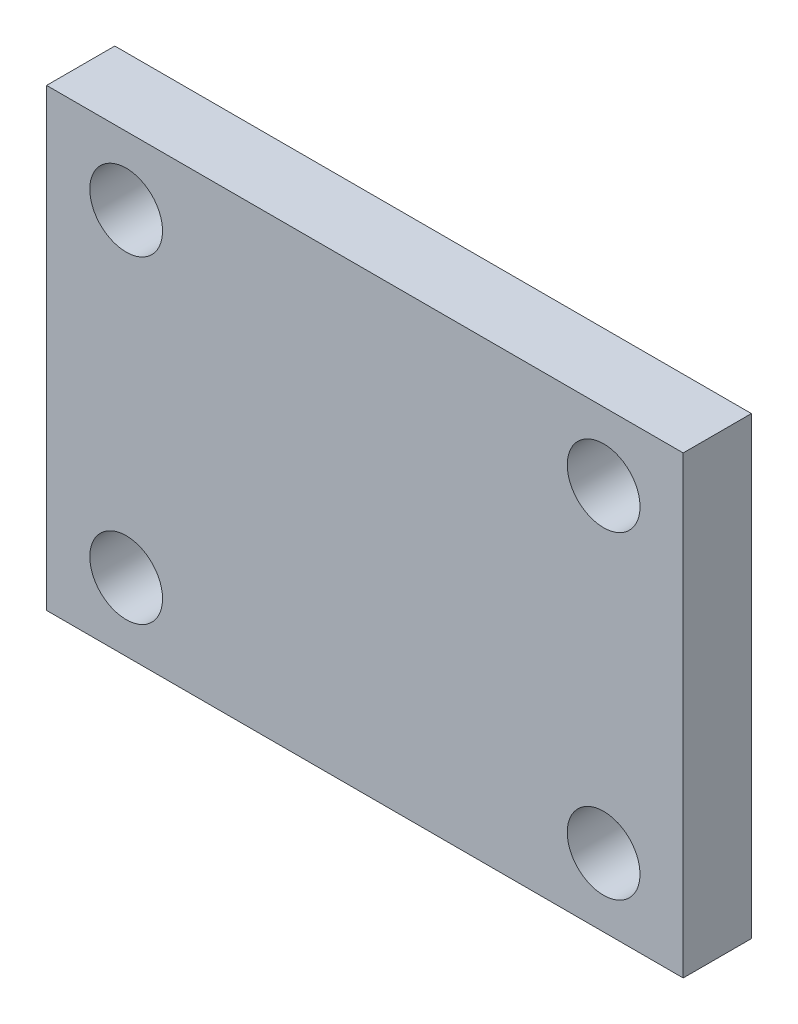
from build123d import *

# Parameters (mm, degrees)
SKETCH1_W           = 28
SKETCH1_H           = 20
SKETCH1_R           = 1.6
BOSS_EXTRUDE1_DEPTH = 1.5


with BuildPart() as part:
    # Sketch1 → Boss-Extrude1 (new, symmetric)
    with BuildSketch(Plane.XY):
        Rectangle(SKETCH1_W, SKETCH1_H)
        with Locations((10.5, 7)):
            Circle(SKETCH1_R, mode=Mode.SUBTRACT)
        with Locations(Location((-10.5, 7, 0), (0, 0, 180))):
            Circle(SKETCH1_R, mode=Mode.SUBTRACT)
        with Locations(Location((10.5, -7, 0), (0, 0, 180))):
            Circle(SKETCH1_R, mode=Mode.SUBTRACT)
        with Locations((-10.5, -7)):
            Circle(SKETCH1_R, mode=Mode.SUBTRACT)
    extrude(amount=BOSS_EXTRUDE1_DEPTH, both=True)


solid = part.part
